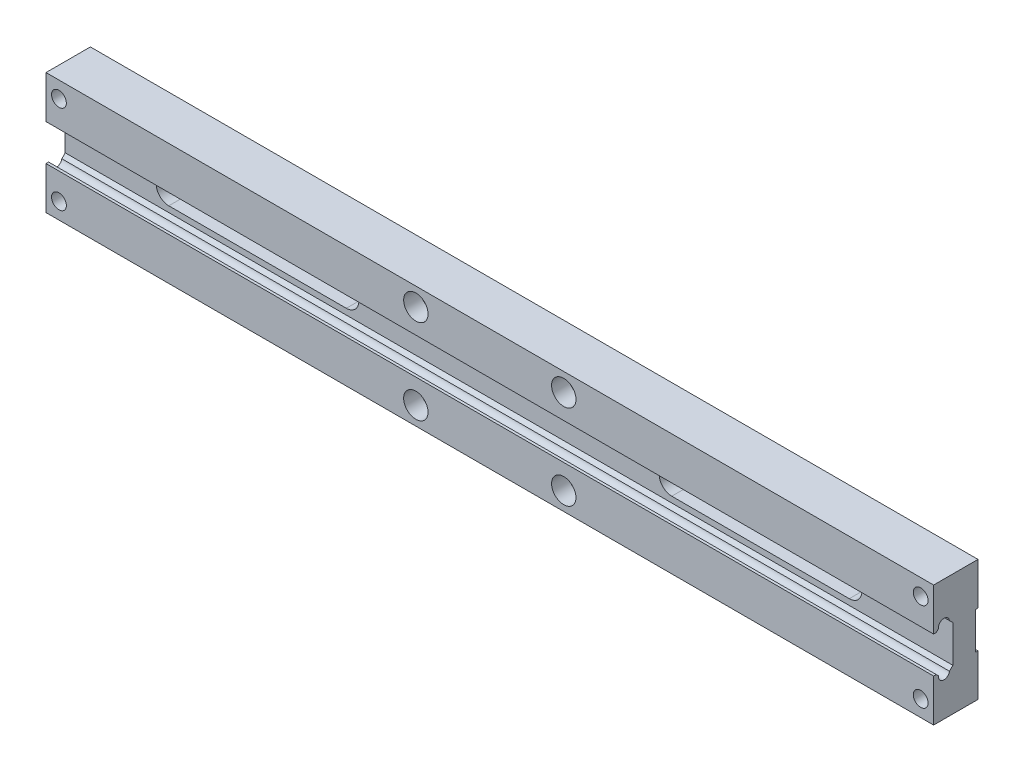
SolidWorks part; units mm, degrees
material "AISI 1045 钢，冷拔"
ref_plane "前视基准面" through (0, 0, 0) normal (0, 0, 1) x (1, 0, 0)
ref_plane "上视基准面" through (0, 0, 0) normal (0, 1, 0) x (1, 0, 0)
ref_plane "右视基准面" through (0, 0, 0) normal (1, 0, 0) x (0, 0, -1)
other "Configuration Table"
sketch "草图1" plane through (0, 0, 0) normal (0, 0, 1) x (1, 0, 0)
  line L1 (-60, -8.2) -> (60, -8.2)
  line L2 (-60, -8.2) -> (-60, 8.2)
  line L3 (-60, 8.2) -> (60, 8.2)
  line L4 (60, -8.2) -> (60, 8.2)
  line L5 (-60, -8.2) -> (60, 8.2) construction
  line L6 (-60, 8.2) -> (60, -8.2) construction
  point P0 (0, 0)
  dimension "D1" = 120
  dimension "D2" = 16.4
extrude "凸台-拉伸1" add sketch "草图1" along normal mid plane 6
sketch "草图2" plane through (0, 0, 3) normal (0, 0, 1) x (1, 0, 0)
  line L1 (60, 8.2) -> (-60, 8.2) construction
  circle A0 centre (-10, 5.75) radius 1.65
  circle A1 centre (-10, 5.75) radius 1
  circle A2 centre (10, 5.75) radius 1
  circle A3 centre (10, 5.75) radius 1.65
  circle A4 centre (10, -5.75) radius 1.65
  circle A5 centre (10, -5.75) radius 1
  circle A6 centre (-10, -5.75) radius 1
  circle A7 centre (-10, -5.75) radius 1.65
  point P16 (0, 0)
  dimension "D1" = 3.3
  dimension "D2" = 2
  dimension "D4" = 2.45
extrude "切除-拉伸2" cut sketch "草图2" against normal blind 2.3
sketch "草图3" plane through (0, 0, 3) normal (0, 0, 1) x (1, 0, 0)
  circle A0 centre (-10, 5.75) radius 1
  circle A1 centre (10, 5.75) radius 1
  circle A2 centre (-10, -5.75) radius 1
  circle A3 centre (10, -5.75) radius 1
  dimension "D1" = 2
  dimension "D2" = 2
  dimension "D3" = 2
  dimension "D4" = 2
extrude "切除-拉伸3" cut sketch "草图3" against normal through all
sketch "草图4" plane through (-60, 0, 0) normal (-1, 0, 0) x (0, 0, 1)
  line L1 (-3, 2.5) -> (-2.65, 2.5)
  line L2 (-2.65, 2.5) -> (-2.65, -2.5)
  line L3 (0.4, -2.5) -> (0.4, 2.5)
  line L4 (-3, 8.2) -> (-3, -8.2)
  line L5 (-3, -8.2) -> (3, -8.2)
  line L6 (3, -8.2) -> (3, 8.2)
  line L7 (3, 8.2) -> (-3, 8.2)
  line L8 (-3, 2.5) -> (-3, -2.5)
  line L9 (-3, -8.2) -> (3, -8.2)
  line L10 (3, -2.4543) -> (3, 2.4543)
  line L11 (3, 8.2) -> (-3, 8.2)
  line L12 (0.4, 2.5) -> (0.8596, 2.9596)
  line L13 (2.65, 2.4543) -> (3, 2.4543)
  line L14 (2.65, 2.4543) -> (2.3459, 2.7583)
  line L15 (2.65, -2.4543) -> (2.3459, -2.7583)
  line L16 (2.65, -2.4543) -> (3, -2.4543)
  line L17 (0.4, -2.5) -> (0.8596, -2.9596)
  line L18 (-3, -2.5) -> (-2.65, -2.5)
  arc A0 (2.3459, 2.7583) -> (0.8596, 2.9596) centre (1.6016, 2.8501) ccw
  arc A1 (2.3459, -2.7583) -> (0.8596, -2.9596) centre (1.6016, -2.8501) cw
  point P25 (0.4, 0)
  point P26 (-2.65, 0)
  dimension "D11" = 1.5
  dimension "D2" = 0.35
  dimension "D3" = 2.5
  dimension "D4" = 2.5
  dimension "D5" = 225
  dimension "D6" = 0.65
  dimension "D7" = 3.05
  dimension "D8" = 135
  dimension "D9" = 0.35
  dimension "D10" = 0.43
  dimension "D1" = 0
extrude "切除-拉伸5" cut sketch "草图4" against normal through all contours L10 L13 L14 A0 L12 L3 L17 A1 L15 L16 | L8 L18 L2 L1
sketch "草图5" plane through (0, 0, 0.4) normal (0, 0, 1) x (1, 0, 0)
  line L0 (-46, 0) -> (-22, 0) construction
  line L1 (-46, 1.7) -> (-22, 1.7)
  line L2 (-46, -1.7) -> (-22, -1.7)
  line L3 (0, 0) -> (0, -4.869) construction
  line L4 (46, 0) -> (22, 0) construction
  line L9 (46, 1.7) -> (22, 1.7)
  line L10 (46, -1.7) -> (22, -1.7)
  arc A0 (-46, 1.7) -> (-46, -1.7) centre (-46, 0) ccw
  arc A1 (-22, -1.7) -> (-22, 1.7) centre (-22, 0) ccw
  arc A6 (46, 1.7) -> (46, -1.7) centre (46, 0) cw
  arc A7 (22, -1.7) -> (22, 1.7) centre (22, 0) cw
  point P3 (-34, 0)
  point P12 (34, 0)
  dimension "D3" = 22
  dimension "D1" = 3.4
  dimension "D2" = 24
extrude "切除-拉伸6" cut sketch "草图5" against normal through all
sketch "草图6" plane through (0, 0, 0.4) normal (0, 0, 1) x (1, 0, 0)
  line L0 (0, 8.2) -> (0, 0) construction
  line L1 (60, 8.2) -> (-60, 8.2) construction
sketch "草图7" plane through (0, 0, -3) normal (0, 0, -1) x (-1, 0, 0)
  circle A0 centre (-58.25, -6) radius 1
  circle A1 centre (-58.25, 6) radius 1
  dimension "D1" = 2
  dimension "D2" = 2
extrude "切除-拉伸7" cut sketch "草图7" against normal through all both and the other way through all
sketch "草图8" plane through (0, 0, 3) normal (0, 0, 1) x (1, 0, 0)
  circle A0 centre (58.25, 6) radius 1
  circle A1 centre (58.25, -6) radius 1
  dimension "D1" = 2
sketch "草图9" plane through (0, 0, 3) normal (0, 0, 1) x (1, 0, 0)
  circle A0 centre (-58.25, 6) radius 1
  circle A1 centre (-58.25, -6) radius 1
  dimension "D1" = 2
extrude "切除-拉伸10" cut sketch "草图9" against normal through all both and the other way through all
